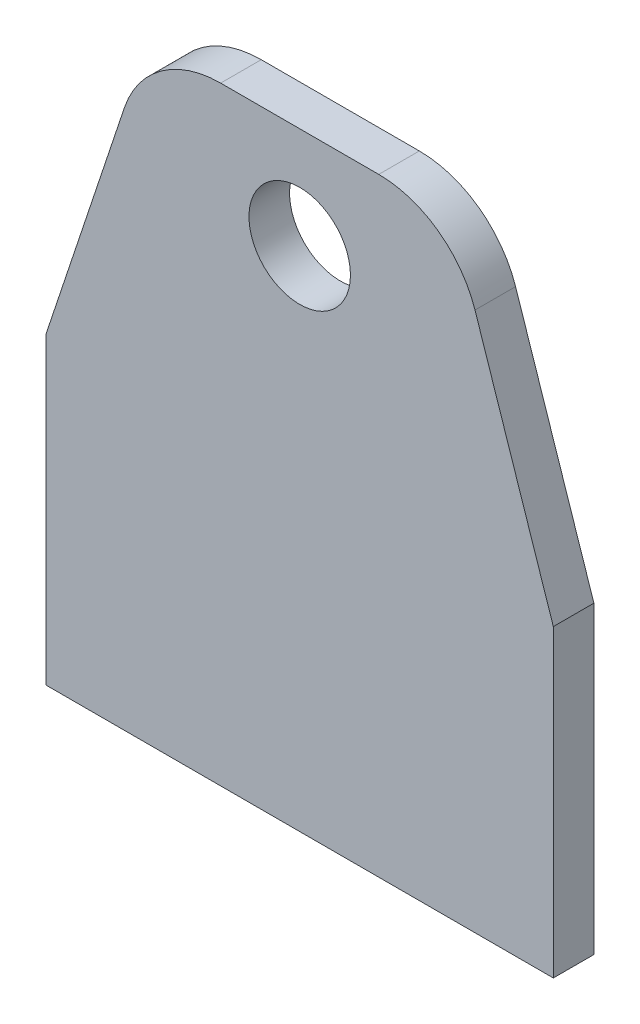
SolidWorks part; units mm, degrees
material "1023 碳钢板 (SS)"
ref_plane "Front Plane" through (0, 0, 0) normal (0, 0, 1) x (1, 0, 0)
ref_plane "Top Plane" through (0, 0, 0) normal (0, 1, 0) x (1, 0, 0)
ref_plane "Right Plane" through (0, 0, 0) normal (1, 0, 0) x (0, 0, -1)
sketch "Sketch1" plane through (0, 0, 0) normal (0, 0, 1) x (1, 0, 0)
  line L2 (33.4332, 28.0778) -> (17.8483, 28.0778)
  line L4 (10.6407, 28.0778) -> (10.6407, -31.9222) construction
  line L5 (10.6407, -31.9222) -> (76.7005, -31.9222) construction
  line L8 (0.6407, -1.9222) -> (50.6407, -1.9222) construction
  line L9 (8.3615, 21.24) -> (0.6407, -1.9222)
  line L10 (42.92, 21.24) -> (50.6407, -1.9222)
  line L11 (0.6407, -1.9222) -> (0.6407, -31.9222)
  line L12 (50.6407, -1.9222) -> (50.6407, -31.9222)
  line L13 (0.6407, -31.9222) -> (50.6407, -31.9222)
  arc A0 (42.92, 21.24) -> (33.4332, 28.0778) centre (33.4332, 18.0778) ccw
  arc A1 (17.8483, 28.0778) -> (8.3615, 21.24) centre (17.8483, 18.0778) ccw
  circle A2 centre (25.6407, 18.0778) radius 5
  point P11 (40.6407, 28.0778)
  point P17 (25.6407, 28.0778)
  dimension "D5" = 10
  dimension "D6" = 10
  dimension "D1" = 30
  dimension "D2" = 60
  dimension "D3" = 30
  dimension "D4" = 10
  dimension "D7" = 20
extrude "Boss-Extrude1" add sketch "Sketch1" along normal blind 4
